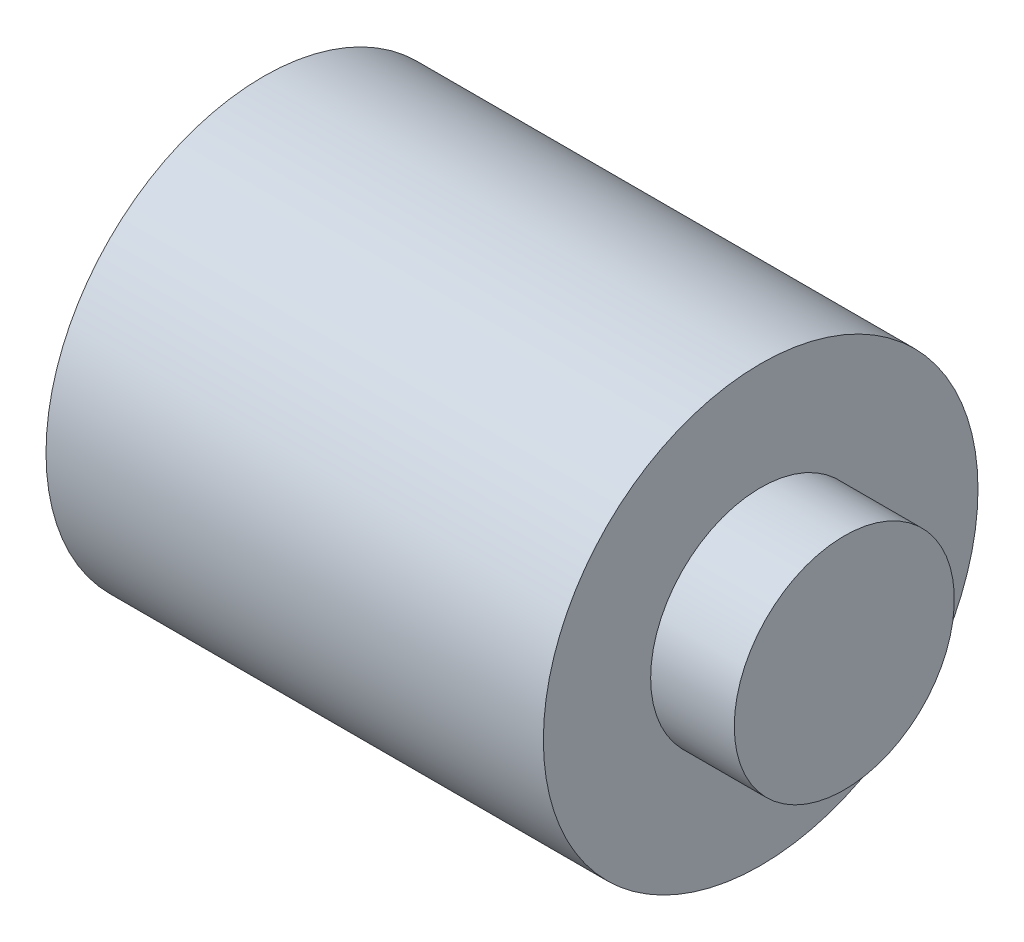
from build123d import *

# Parameters (mm, degrees)
SKETCH_1_R      = 19.75
EXTRUDE_1_DEPTH = 45.2
SKETCH_2_R      = 10
EXTRUDE_2_DEPTH = 7.6


with BuildPart() as part:
    # 草图1 → 凸台-拉伸1 (new body)
    with BuildSketch(Plane(origin=(0, 0, 0), x_dir=(0, 0, -1), z_dir=(1, 0, 0))):
        Circle(SKETCH_1_R)
    extrude(amount=EXTRUDE_1_DEPTH)

    # 草图2 → 凸台-拉伸2 (add)
    with BuildSketch(Plane(origin=(45.2, 0, 0), x_dir=(0, 0, -1), z_dir=(1, 0, 0))):
        with Locations(Location((0, 0, 0), (0, 0, 180))):
            Circle(SKETCH_2_R)
    extrude(amount=EXTRUDE_2_DEPTH)


solid = part.part
